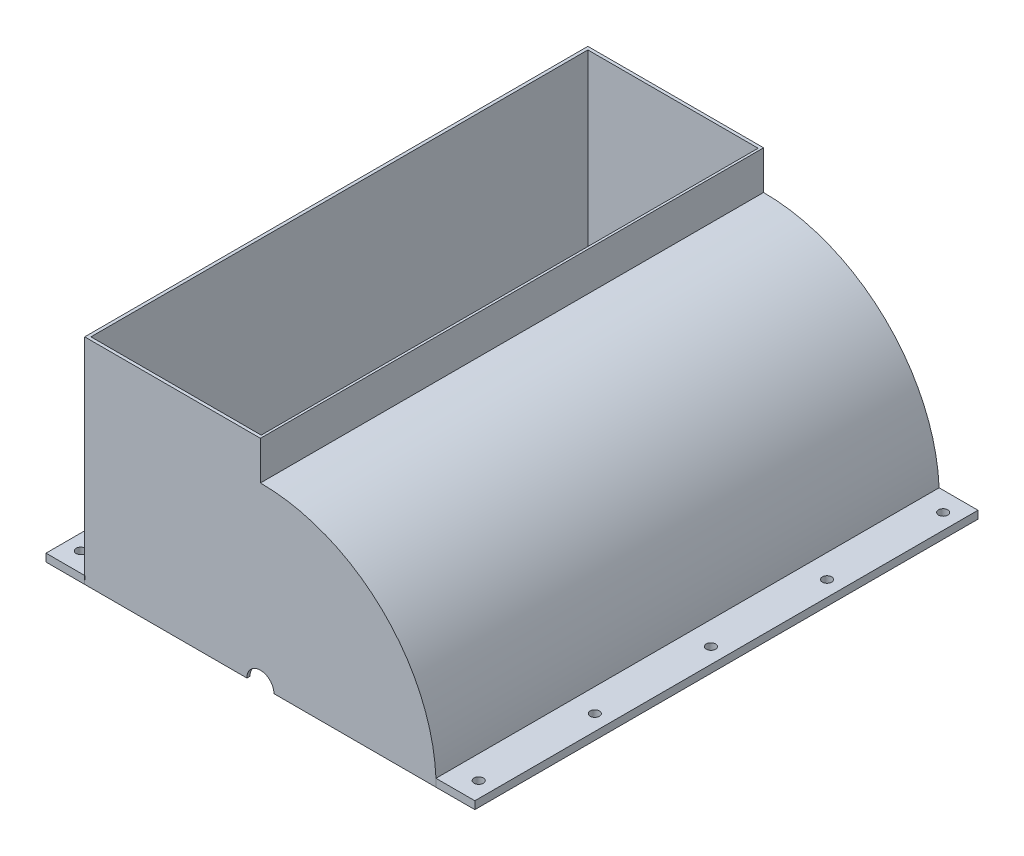
SolidWorks part; units mm, degrees
material "AISI 304"
ref_plane "Front Plane" through (0, 0, 0) normal (0, 0, 1) x (1, 0, 0)
ref_plane "Top Plane" through (0, 0, 0) normal (0, 1, 0) x (1, 0, 0)
ref_plane "Right Plane" through (0, 0, 0) normal (1, 0, 0) x (0, 0, -1)
other "Configuration Table"
sketch "Sketch1" plane through (0, 0, 0) normal (0, 0, 1) x (1, 0, 0)
  line L0 (-227, 0) -> (-227, 377)
  line L1 (-227, 377) -> (0, 377)
  line L2 (0, 377) -> (0, 227)
  line L3 (-223, 0) -> (-223, 377)
  line L4 (-3, 377) -> (-3, 226.9802)
  line L5 (-227, 0) -> (227, 0) construction
  line L6 (227, 0) -> (227, -180)
  line L7 (227, -180) -> (-50, -280.8198)
  line L8 (223, 0) -> (223, -177.1992)
  line L9 (223, -177.1992) -> (-51.3681, -277.061)
  line L10 (-51.3681, -277.061) -> (-50, -280.8198)
  line L11 (-113.5, -196.5878) -> (-60, -227.476)
  line L12 (-111.5, -193.1237) -> (-58, -224.0119)
  line L13 (-58, -224.0119) -> (-60, -227.476)
  line L14 (-227, 0) -> (-277, 0) construction
  line L15 (227, 0) -> (277, 0) construction
  line L16 (-50, -280.8198) -> (330.4492, -280.8198) construction
  line L17 (-277, 0) -> (-223, 0)
  line L18 (-277, 0) -> (-277, 10)
  line L19 (-277, 10) -> (-223, 10)
  line L20 (-223, 0) -> (-223, 10)
  line L21 (277, 0) -> (226.7796, 0)
  line L22 (277, 0) -> (277, 10)
  line L23 (277, 10) -> (226.7796, 10)
  line L24 (226.7796, 0) -> (226.7796, 10)
  line L25 (-277, 0) -> (-226.9207, 0)
  line L26 (-277, 0) -> (-277, -6)
  line L27 (-277, -6) -> (-226.9207, -6)
  line L28 (-226.9207, 0) -> (-226.9207, -6)
  line L29 (277, 0) -> (223, 0)
  line L30 (277, 0) -> (277, -6)
  line L31 (277, -6) -> (223, -6)
  line L32 (223, 0) -> (223, -6)
  line L33 (-226.9207, -6) -> (-232.9207, -6)
  line L34 (-226.9207, -6) -> (-226.9207, -227.476)
  line L35 (-226.9207, -227.476) -> (-232.9207, -227.476)
  line L36 (-232.9207, -6) -> (-232.9207, -227.476)
  line L37 (233, -6) -> (227, -6)
  line L38 (233, -6) -> (233, -227.476)
  line L39 (233, -227.476) -> (227, -227.476)
  line L40 (227, -6) -> (227, -227.476)
  line L41 (-60, -227.476) -> (-291.314, -227.476) construction
  line L42 (-60, -227.476) -> (-226.9207, -227.476)
  line L43 (233, -227.476) -> (277, -227.476)
  line L44 (233, -227.476) -> (233, -221.476)
  line L45 (233, -221.476) -> (277, -221.476)
  line L46 (277, -227.476) -> (277, -221.476)
  line L47 (-232.9207, -227.476) -> (-276.9207, -227.476)
  line L48 (-232.9207, -227.476) -> (-232.9207, -221.476)
  line L49 (-232.9207, -221.476) -> (-276.9207, -221.476)
  line L50 (-276.9207, -227.476) -> (-276.9207, -221.476)
  line L51 (-3, 226.9802) -> (-3, 212.6706)
  line L52 (0, 227) -> (0, 212.6706)
  circle A0 centre (0, 0) radius 208
  circle A1 centre (0, 0) radius 223
  circle A2 centre (0, 0) radius 227
  dimension "D1" = 416
  dimension "D4" = 150
  dimension "D5" = 3
  dimension "D6" = 180
  dimension "D7" = 110
  dimension "D8" = 50
  dimension "D10" = 30
  dimension "D11" = 60
  dimension "D12" = 4
  dimension "D13" = 50
  dimension "D14" = 50
  dimension "D15" = 10
  dimension "D16" = 10
  dimension "D17" = 6
  dimension "D18" = 6
  dimension "D19" = 6
  dimension "D20" = 6
  dimension "D21" = 0
  dimension "D22" = 0
  dimension "D23" = 44
  dimension "D24" = 6
  dimension "D25" = 6
  dimension "D26" = 44
  dimension "D2" = 15
  dimension "D3" = 4
  dimension "D9" = 4
extrude "Boss-Extrude1" add sketch "Sketch1" along normal mid plane 650 contours L19 L18 L17 L0 | L19 A2 L17 L3 | L3 A2 L19 | A2 L3 L1 L0 L19 | A2 L2 L1 L4 | L52 A2 L51 A1 | L24 A2 L52 A1 L29 | A2 L21 L22 L23
sketch "Sketch3" plane through (0, 0, 325) normal (0, 0, 1) x (1, 0, 0)
  line L0 (-3, 377) -> (-3, 222.9798) construction
  line L1 (-3, 377) -> (-3, 222.9798)
  line L2 (-223, 377) -> (-3, 377)
  line L3 (-223, 0) -> (223, 0)
  line L5 (-223, 0) -> (-223, 377)
  line L6 (-223, 377) -> (-227, 377)
  line L7 (-227, 377) -> (-227, 10)
  line L8 (-227, 10) -> (-226.7796, 10)
  line L9 (-227, 0) -> (-223, 0)
  line L10 (-223, 0) -> (-223, 377)
  line L11 (-223, 377) -> (-227, 377)
  line L12 (-227, 377) -> (-227, 10)
  line L13 (-227, 10) -> (-226.7796, 10)
  line L14 (-227, 0) -> (-223, 0)
  arc A0 (223, 0) -> (-3, 222.9798) centre (0, 0) ccw construction
  arc A1 (-226.7796, 10) -> (-227, 0) centre (0, 0) ccw
  arc A2 (-226.7796, 10) -> (-227, 0) centre (0, 0) ccw
  arc A3 (223, 0) -> (-3, 222.9798) centre (0, 0) ccw
  line M7 (-223, 0) -> (-223, 377)
  dimension "D1" = 0
extrude "Boss-Extrude4" add sketch "Sketch3" against normal blind 4 contours L3 A3 L1 L2 M7
sketch "Sketch4" plane through (0, 0, -325) normal (0, 0, -1) x (-1, 0, 0)
  line L0 (223, 0) -> (223, 377) construction
  line L1 (223, 0) -> (223, 377)
  line L2 (3, 377) -> (223, 377)
  line L3 (-223, 0) -> (223, 0)
  line L5 (3, 222.9798) -> (3, 377)
  line L6 (3, 377) -> (0, 377)
  line L7 (0, 377) -> (0, 227)
  line L8 (-226.7796, 10) -> (-226.7796, 0)
  line L9 (-226.7796, 0) -> (-223, 0)
  line L10 (3, 222.9798) -> (3, 377)
  line L11 (3, 377) -> (0, 377)
  line L12 (0, 377) -> (0, 227)
  line L13 (-226.7796, 10) -> (-226.7796, 0)
  line L14 (-226.7796, 0) -> (-223, 0)
  arc A2 (0, 227) -> (-226.7796, 10) centre (0, 0) ccw
  arc A3 (3, 222.9798) -> (-223, 0) centre (0, 0) ccw
  arc A4 (0, 227) -> (-226.7796, 10) centre (0, 0) ccw
  arc A5 (3, 222.9798) -> (-223, 0) centre (0, 0) ccw
  line M8 (3, 222.9798) -> (3, 377)
  arc M14 (-223, 0) -> (3, 222.9798) centre (0, 0) cw
  dimension "D1" = 0
extrude "Boss-Extrude5" add sketch "Sketch4" against normal blind 4 contours L3 L1 L2 M14 M8
sketch "Sketch6" plane through (0, 0, 0) normal (0, -1, 0) x (1, 0, 0)
  line L0 (-257, 325) -> (-257, -325) construction
  line L1 (-277, 325) -> (-227, 325) construction
  line L2 (-277, -325) -> (-227, -325) construction
  line L3 (-277, 325) -> (-277, -325) construction
  line L4 (257, 325) -> (257, -325) construction
  line L5 (277, 325) -> (227, 325) construction
  line L6 (277, -325) -> (227, -325) construction
  line L7 (277, 325) -> (277, -325) construction
  circle A0 centre (257, 0) radius 6
  circle A1 centre (-257, 0) radius 6
  dimension "D3" = 12
  dimension "D4" = 12
  dimension "D1" = 20
  dimension "D2" = 20
extrude "Cut-Extrude1" cut sketch "Sketch6" against normal through all both and the other way through all
pattern_linear "LPattern1" count 3 spacing 150 along (0, 0, -1) of "Cut-Extrude1"
pattern_linear "LPattern2" count 3 spacing 150 along (0, 0, 1) of "Cut-Extrude1"
sketch "Sketch7" plane through (0, 0, 325) normal (0, 0, 1) x (1, 0, 0)
  circle A0 centre (0, 0) radius 17.5
  dimension "D1" = 35
extrude "Cut-Extrude2" cut sketch "Sketch7" against normal through all both and the other way through all
sketch "Sketch8" plane through (0, 377, 0) normal (0, 1, 0) x (1, 0, 0)
  line L1 (364.5625, 380.7185) -> (-356.1977, 380.7185)
  line L2 (364.5625, 380.7185) -> (364.5625, -380.7185)
  line L3 (364.5625, -380.7185) -> (-356.1977, -380.7185)
  line L4 (-356.1977, 380.7185) -> (-356.1977, -380.7185)
  line L5 (364.5625, 380.7185) -> (-356.1977, -380.7185) construction
  line L6 (364.5625, -380.7185) -> (-356.1977, 380.7185) construction
  point P0 (4.1824, 0)
extrude "Cut-Extrude3" cut sketch "Sketch8" against normal blind 100
